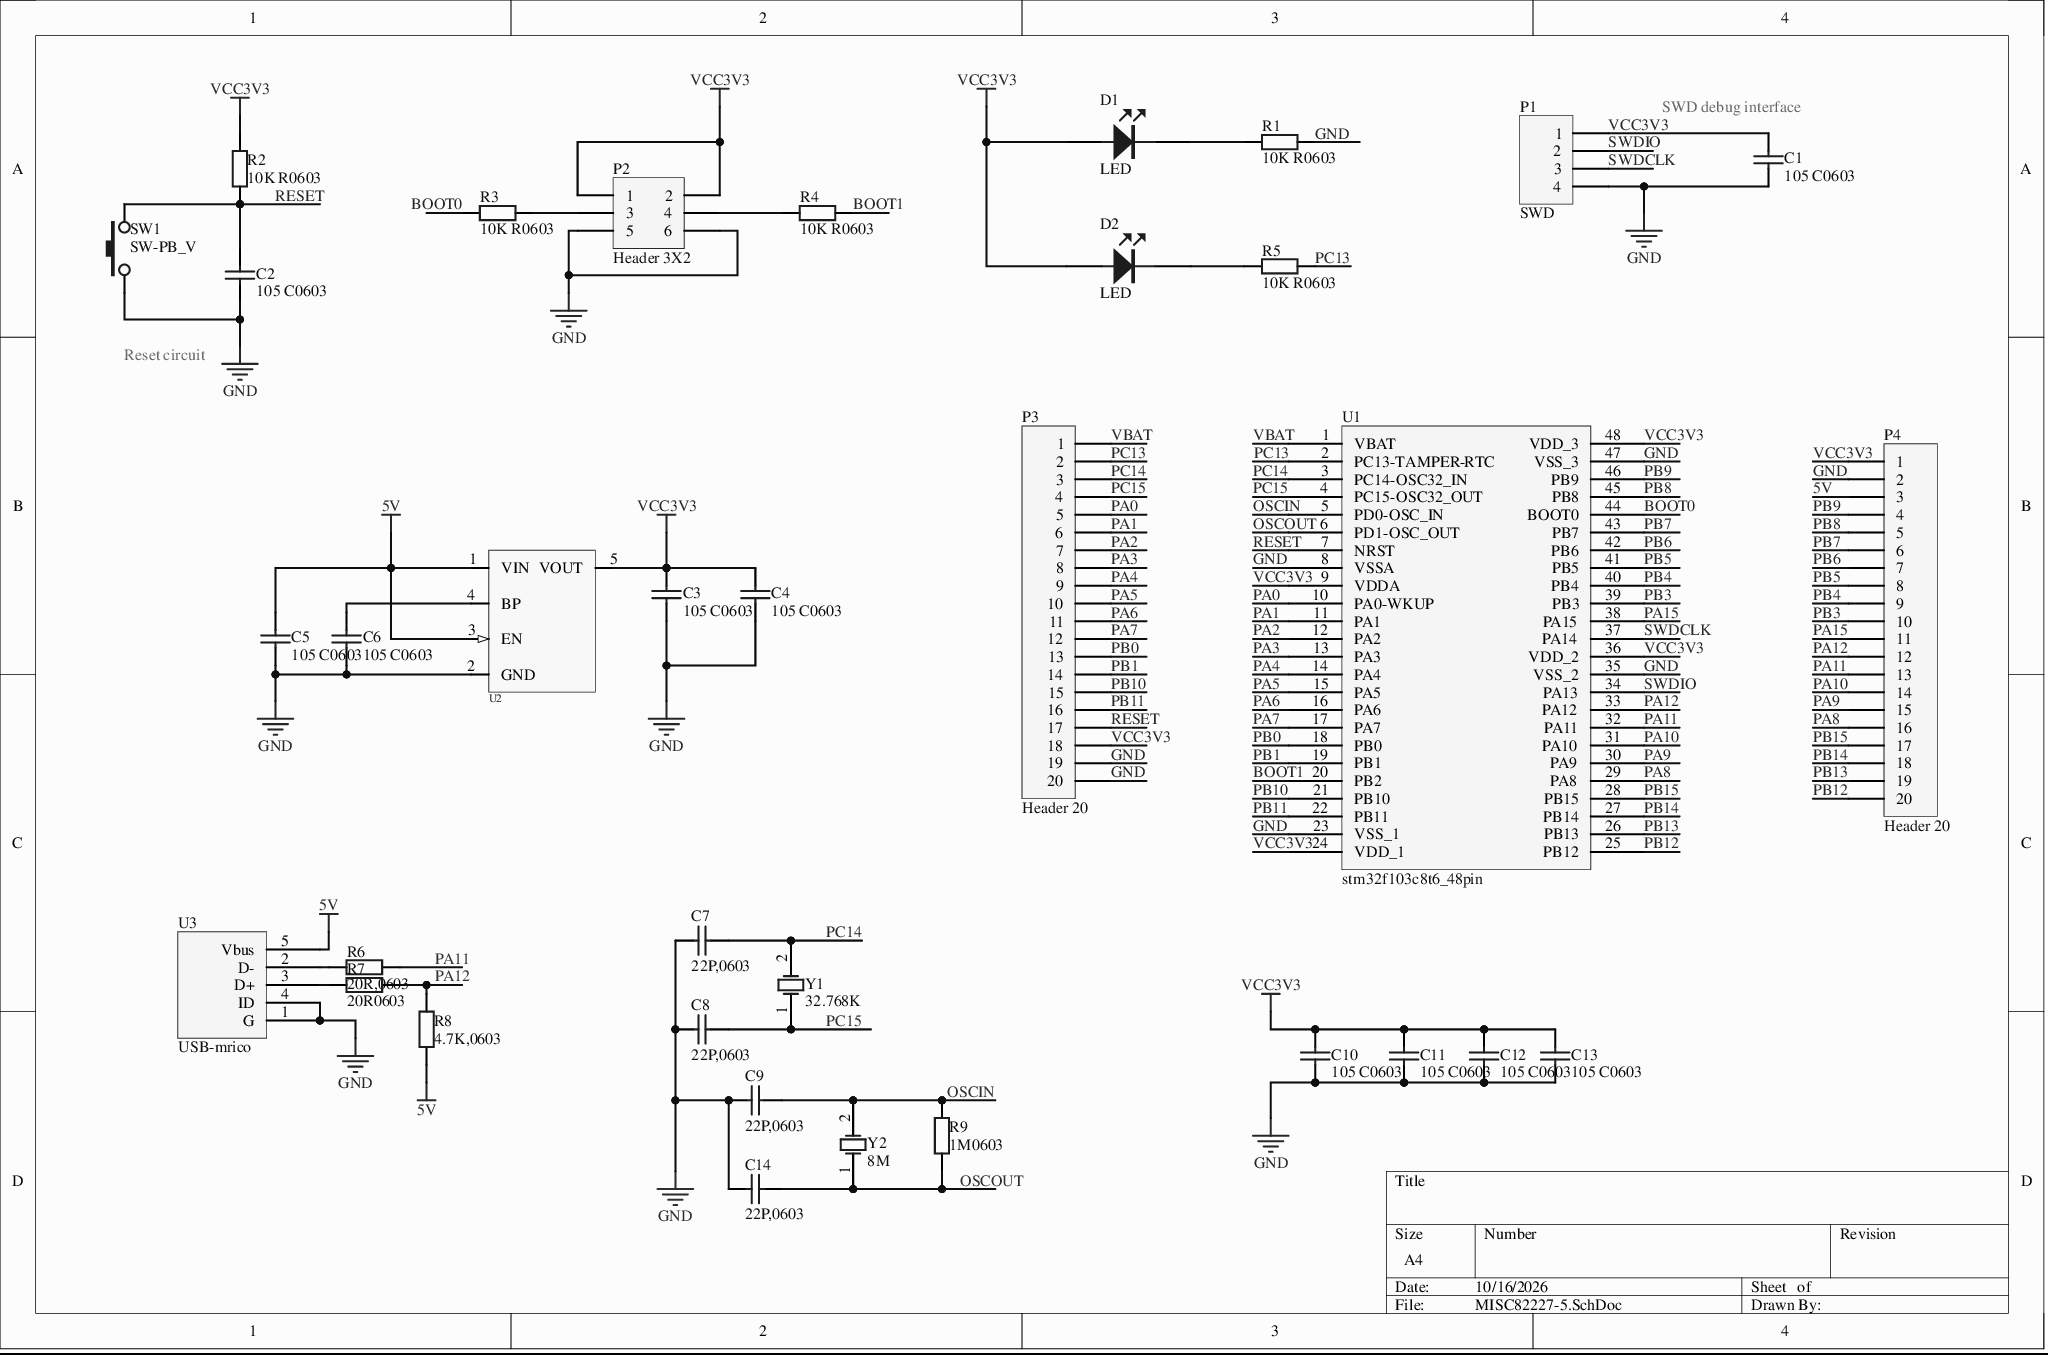
[diagram p0: MISC82227-5.SchDoc]
# Altium project MISC82227-2.PrjPcb
1 sheet, 35 parts. Net scope: global (net labels, ports and power ports of the same name join across sheets).
Board file: MISC82227.PcbDoc

## Sheet MISC82227-5.SchDoc
size A4

### Parts
C1  105 C0603  [C 0603]
C2  105 C0603  [C 0603]
C3  105 C0603  [C 0603]
C4  105 C0603  [C 0603]
C5  105 C0603  [C 0603]
C6  105 C0603  [C 0603]
C7  22P,0603  [C 0603]
C8  22P,0603  [C 0603]
C9  22P,0603  [C 0603]
C10  105 C0603  [C 0603]
C11  105 C0603  [C 0603]
C12  105 C0603  [C 0603]
C13  105 C0603  [C 0603]
C14  22P,0603  [C 0603]
D1  LED  [LED 0805G]
D2  LED  [LED 0805G]
P1  SWD  [HDR-1X4_H]
P2  Header 3X2  [HDR-3X2]
P3  Header 20  [HDR1X20]
P4  Header 20  [HDR1X20]
R1  10K R0603  [R 0603]
R2  10K R0603  [R 0603]
R3  10K R0603  [R 0603]
R4  10K R0603  [R 0603]
R5  10K R0603  [R 0603]
R6  20R,0603  [R 0603]
R7  20R0603  [R 0603]
R8  4.7K,0603  [R 0603]
R9  1M0603  [R 0603]
SW1  SW-PB_V  [TSW SMD-3*6*2.5]
U1  stm32f103c8t6_48pin  [TQFP48 7x7_L]
U2  RT9193  [SOT23-5L]  (value not drawn)
U3  USB-mrico  [USB-micro_B]
Y1  32.768K  [XTAL-49S DIP]
Y2  8M  [XTAL-49S DIP]

### Nets
5V: C5.2 P4.3 R8.1 U2.1(VIN) U2.3(EN) U3.5(Vbus)
GND: C1.1 C2.1 C3.1 C4.1 C5.1 C6.1 C7.2 C8.2 C9.2 C10.1 C11.1 C12.1 C13.1 C14.2 P1.4 P2.5 P2.6 P3.19 P3.20 P4.2 R1.2 SW1.1 U1.8(VSSA) U1.23(VSS_1) U1.35(VSS_2) U1.47(VSS_3) U2.2(GND) U3.1(G) U3.4(ID)
VCC3V3: C1.2 C3.2 C4.2 C10.2 C11.2 C12.2 C13.2 D1.1 D2.1 P1.1 P2.1 P2.2 P3.18 P4.1 R2.2 U1.9(VDDA) U1.24(VDD_1) U1.36(VDD_2) U1.48(VDD_3) U2.5(VOUT)
BOOT0: R3.1 U1.44(BOOT0)
BOOT1: R4.2 U1.20(PB2)
OSCIN: C9.1 R9.2 U1.5(PD0-OSC_IN) Y2.2(OSC2)
OSCOUT: C14.1 R9.1 U1.6(PD1-OSC_OUT) Y2.1(OSC1)
PA0: P3.5 U1.10(PA0-WKUP)
PA1: P3.6 U1.11(PA1)
PA2: P3.7 U1.12(PA2)
PA3: P3.8 U1.13(PA3)
PA4: P3.9 U1.14(PA4)
PA5: P3.10 U1.15(PA5)
PA6: P3.11 U1.16(PA6)
PA7: P3.12 U1.17(PA7)
PA8: P4.16 U1.29(PA8)
PA9: P4.15 U1.30(PA9)
PA10: P4.14 U1.31(PA10)
PA11: P4.13 R6.2 U1.32(PA11)
PA12: P4.12 R7.2 R8.2 U1.33(PA12)
PA15: P4.11 U1.38(PA15)
PB0: P3.13 U1.18(PB0)
PB1: P3.14 U1.19(PB1)
PB3: P4.10 U1.39(PB3)
PB4: P4.9 U1.40(PB4)
PB5: P4.8 U1.41(PB5)
PB6: P4.7 U1.42(PB6)
PB7: P4.6 U1.43(PB7)
PB8: P4.5 U1.45(PB8)
PB9: P4.4 U1.46(PB9)
PB10: P3.15 U1.21(PB10)
PB11: P3.16 U1.22(PB11)
PB12: P4.20 U1.25(PB12)
PB13: P4.19 U1.26(PB13)
PB14: P4.18 U1.27(PB14)
PB15: P4.17 U1.28(PB15)
PC13: P3.2 R5.2 U1.2(PC13-TAMPER-RTC)
PC14: C7.1 P3.3 U1.3(PC14-OSC32_IN) Y1.2(OSC2)
PC15: C8.1 P3.4 U1.4(PC15-OSC32_OUT) Y1.1(OSC1)
RESET: C2.2 P3.17 R2.1 SW1.2 U1.7(NRST)
SWDCLK: P1.3 U1.37(PA14)
SWDIO: P1.2 U1.34(PA13)
VBAT: P3.1 U1.1(VBAT)
NetC6_2: C6.2 U2.4(BP)
NetD1_2: D1.2 R1.1
NetD2_2: D2.2 R5.1
NetP2_3: P2.3 R3.2
NetP2_4: P2.4 R4.1
NetR6_1: R6.1 U3.2(D-)
NetR7_1: R7.1 U3.3(D+)

### Notes on the sheet
- (near C1) SWD debug interface
- Reset circuit

### Library data of the parts
C1-C6 C10-C13 = Cap: Value: 104; Published: 8-Jun-2000; LatestRevisionDate: 17-Jul-2002; LatestRevisionNote: Re-released for DXP Platform.; Publisher: Altium Limited
C7-C9 C14 = Cap: Capacitor; Value: 104; Published: 8-Jun-2000; LatestRevisionDate: 17-Jul-2002; LatestRevisionNote: Re-released for DXP Platform.; Publisher: Altium Limited
P1 = Header 4: Header, 4-Pin; LatestRevisionDate: 17-Jul-2002; LatestRevisionNote: Re-released for DXP Platform.; Publisher: Altium Limited
P2 = Header 3X2: Header, 3-Pin, Dual row; LatestRevisionDate: 17-Jul-2002; LatestRevisionNote: Re-released for DXP Platform.; Publisher: Altium Limited
P3 P4 = Header 20: Header, 20-Pin; LatestRevisionDate: 17-Jul-2002; LatestRevisionNote: Re-released for DXP Platform.; Publisher: Altium Limited
R1-R5 = Res2: Published: 8-Jun-2000; LatestRevisionDate: 17-Jul-2002; LatestRevisionNote: Re-released for DXP Platform.; Publisher: Altium Limited
R6-R9 = Res2: Resistor; Published: 8-Jun-2000; LatestRevisionDate: 17-Jul-2002; LatestRevisionNote: Re-released for DXP Platform.; Publisher: Altium Limited
U2 = RT9193X_5P: ICA_MFR_NAME: RICHTEK; ICA_PARTNUM: $$2191094$$RT9193-15CU5; Part Number: TMP-13
U3 = usb-STM
Y1 Y2 = XTAL: Crystal Oscillator; Published: 8-Jun-2000; LatestRevisionDate: 17-Jul-2002; LatestRevisionNote: Re-released for DXP Platform.; Publisher: Altium Limited